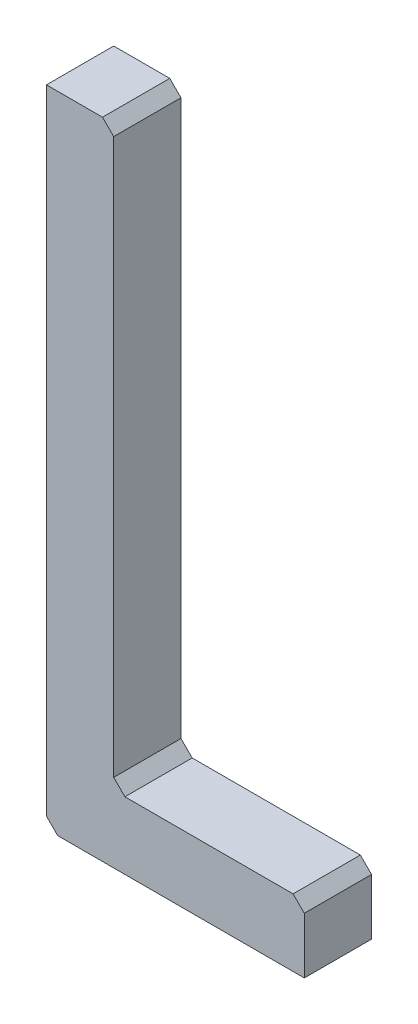
SolidWorks part; units mm, degrees
ref_plane "前视基准面" through (0, 0, 0) normal (0, 0, 1) x (1, 0, 0)
ref_plane "上视基准面" through (0, 0, 0) normal (0, 1, 0) x (1, 0, 0)
ref_plane "右视基准面" through (0, 0, 0) normal (1, 0, 0) x (0, 0, -1)
sketch "草图1" plane through (0, 0, 0) normal (0, 0, 1) x (1, 0, 0)
  line L0 (0, 0) -> (0, 115)
  line L1 (0, 115) -> (12, 115)
  line L2 (12, 115) -> (12, 12)
  line L3 (12, 12) -> (46, 12)
  line L4 (46, 12) -> (46, 0)
  line L5 (46, 0) -> (0, 0)
  dimension "D1" = 115
  dimension "D2" = 46
  dimension "D3" = 12
  dimension "D4" = 12
extrude "凸台-拉伸1" add sketch "草图1" along normal mid plane 12
chamfer "倒角1" distance 2 angle 45 1 edges at (12, 12, 0)
chamfer "倒角2" distance 2 angle 45 1 edges at (0, 0, 0)
chamfer "倒角3" distance 2 angle 45 2 edges at (46, 12, 0) (12, 115, 0)
